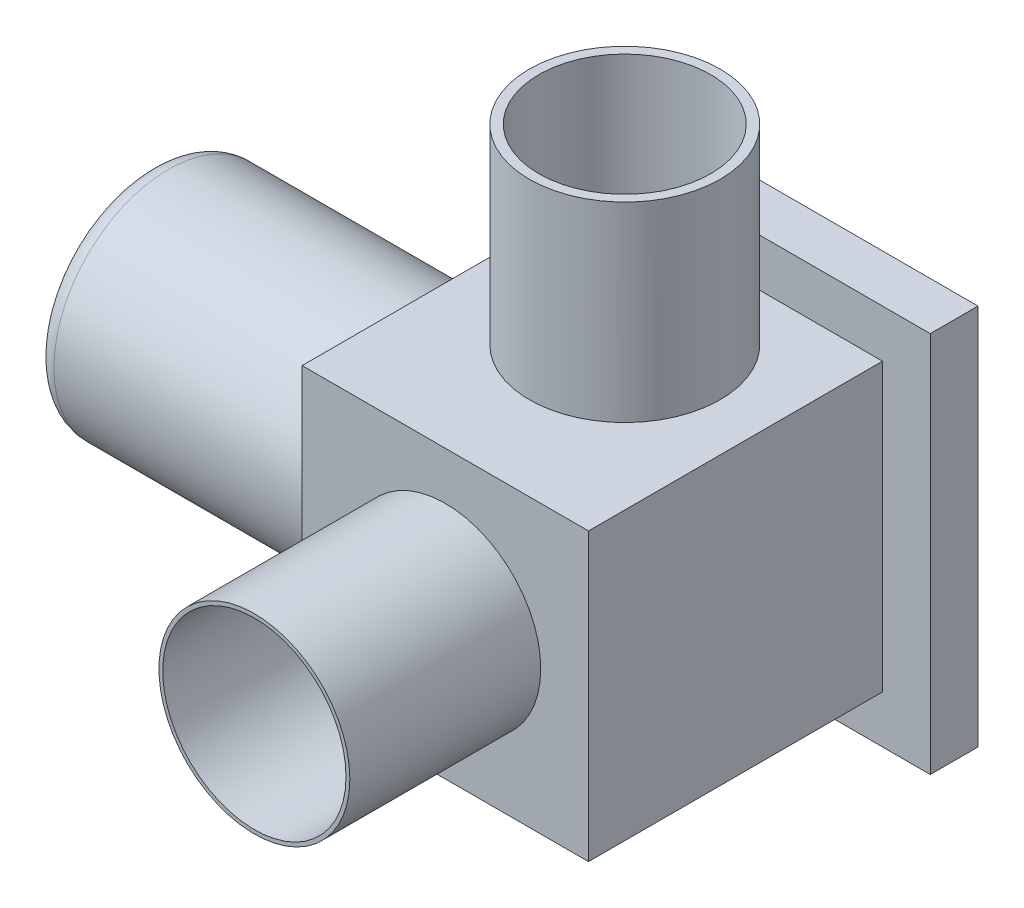
from build123d import *

# Parameters (mm, degrees)
SKETCH_1_W          = 200
SKETCH_1_H          = 200
EXTRUDE_1_DEPTH     = 25
SKETCH_2_W          = 150
SKETCH_2_H          = 150
EXTRUDE_2_DEPTH     = 154
SKETCH_3_R          = 60
EXTRUDE_3_DEPTH     = 154
FILLET_1_R          = 10
SKETCH_4_R          = 50
EXTRUDE_4_DEPTH     = 100
SKETCH_5_R          = 50
SKETCH_5_R_2        = 45
EXTRUDE_5_DEPTH     = 100
SKETCH_6_R          = 48
CUT_EXTRUDE_1_DEPTH = 100


with BuildPart() as part:
    # 草图1 → 凸台-拉伸1 (new body)
    with BuildSketch(Plane.XY):
        Rectangle(SKETCH_1_W, SKETCH_1_H)
    extrude(amount=EXTRUDE_1_DEPTH)

    # 草图2 → 凸台-拉伸2 (add)
    with BuildSketch(Plane.XY.offset(25)):
        Rectangle(SKETCH_2_W, SKETCH_2_H)
    extrude(amount=EXTRUDE_2_DEPTH)

    # 草图3 → 凸台-拉伸3 (add)
    with BuildSketch(Plane(origin=(-75, 0, 0), x_dir=(0, 0, -1), z_dir=(1, 0, 0))):
        with Locations((-105, -5)):
            Circle(SKETCH_3_R)
    extrude(amount=-EXTRUDE_3_DEPTH)

    # 圆角1
    fillet_1_edges = [part.edges().sort_by_distance(p)[0] for p in [
        (-229, -5, 165),
    ]]
    fillet(fillet_1_edges, radius=FILLET_1_R)

    # 草图4 → 凸台-拉伸4 (add)
    with BuildSketch(Plane.XY.offset(179)):
        Circle(SKETCH_4_R)
    extrude(amount=EXTRUDE_4_DEPTH)

    # 草图5 → 凸台-拉伸5 (add)
    with BuildSketch(Plane(origin=(0, 75, 0), x_dir=(1, 0, 0), z_dir=(0, 1, 0))):
        with Locations(Location((0, -85, 0), (0, 0, 90))):
            Circle(SKETCH_5_R)
        with Locations(Location((0, -85, 0), (0, 0, 270))):
            Circle(SKETCH_5_R_2, mode=Mode.SUBTRACT)
    extrude(amount=EXTRUDE_5_DEPTH)

    # 草图6 → 切除-拉伸1 (cut)
    with BuildSketch(Plane.XY.offset(279)):
        Circle(SKETCH_6_R)
    extrude(amount=-CUT_EXTRUDE_1_DEPTH, mode=Mode.SUBTRACT)


solid = part.part
